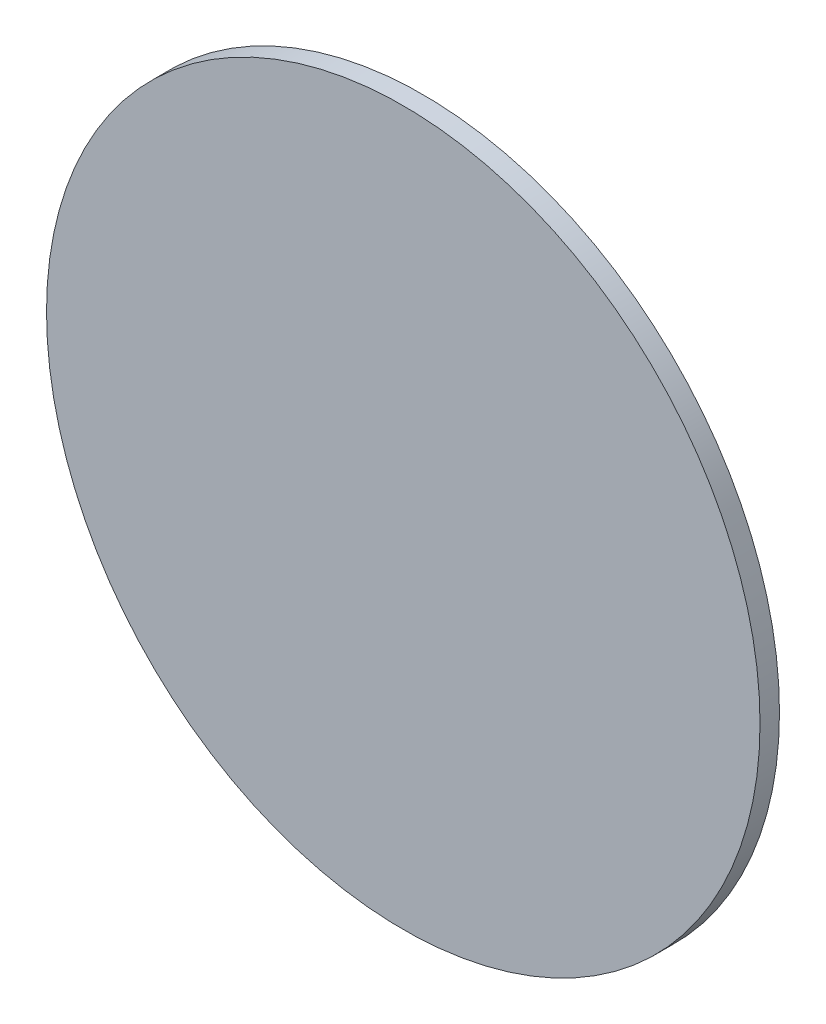
SolidWorks part; units mm, degrees
material "Q235B"
ref_plane "Front Plane" through (0, 0, 0) normal (0, 0, 1) x (1, 0, 0)
ref_plane "Top Plane" through (0, 0, 0) normal (0, 1, 0) x (1, 0, 0)
ref_plane "Right Plane" through (0, 0, 0) normal (1, 0, 0) x (0, 0, -1)
sketch "Sketch1" plane through (0, 0, 0) normal (0, 0, 1) x (1, 0, 0)
  circle A0 centre (0, 0) radius 110
extrude "Boss-Extrude1" add sketch "Sketch1" along normal blind 6
